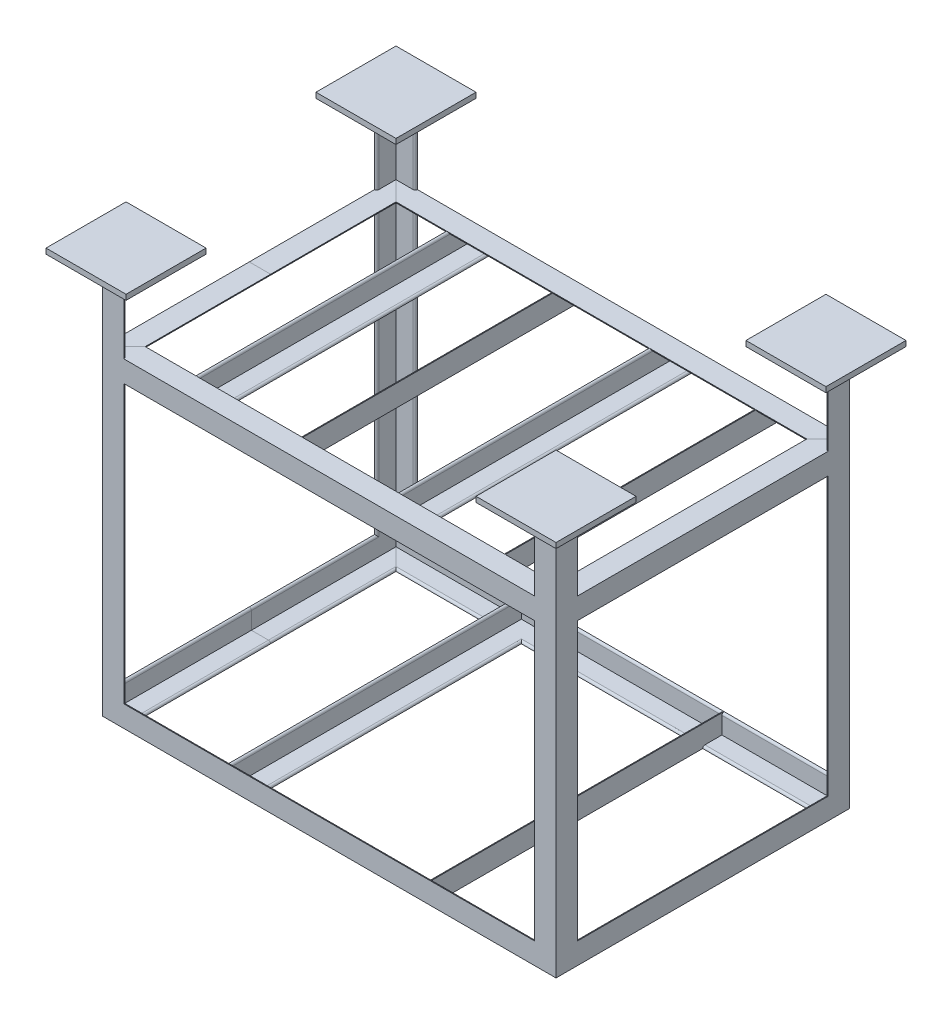
from build123d import *

# Parameters (mm, degrees)
BOSS_EXTRUDE_1_DEPTH = 300
BOSS_EXTRUDE_START   = 150
BOSS_EXTRUDE_2_DEPTH = 150
SKETCH_4_W           = 150
SKETCH_4_H           = 150
BOSS_EXTRUDE_3_DEPTH = 10
BOSS_EXTRUDE_4_REACH = 977.753


with BuildPart() as part:
    # Sweep 1: sweep along a path in Sketch 1
    with BuildLine(Plane(origin=(0, 0, 0), x_dir=(1, 0, 0), z_dir=(0, 1, 0))) as sweep_1_path:
        Line((-425, -275), (-425, 275))
        Line((-425, 275), (425, 275))
        Line((425, 275), (425, -275))
        Line((425, -275), (-425, -275))
    # Sketch 2 → Sweep 1 (sweep)
    with BuildSketch(Plane.XY):
        with BuildLine():
            Line((-425, 0), (-385, 0))
            ThreePointArc((-385, 0), (-386.171572875, -2.828427125), (-389, -4))
            Line((-389, -4), (-421, -4))
            Line((-421, -4), (-421, -36))
            ThreePointArc((-421, -36), (-422.171572875, -38.828427125), (-425, -40))
            Line((-425, -40), (-425, 0))
        make_face()
    sweep(path=sweep_1_path.line, transition=Transition.RIGHT)

    # Sketch 3_2 → Boss-Extrude 1 (add)
    with BuildSketch(Plane(origin=(0, 0, 0), x_dir=(1, 0, 0), z_dir=(0, 1, 0))):
        with BuildLine():
            Line((425, 275), (425, 235))
            ThreePointArc((425, 235), (422.171572875, 236.171572875), (421, 239))
            Line((421, 239), (421, 271))
            Line((421, 271), (389, 271))
            ThreePointArc((389, 271), (386.171572875, 272.171572875), (385, 275))
            Line((385, 275), (425, 275))
        make_face()
        with BuildLine():
            Line((425, -275), (385, -275))
            ThreePointArc((385, -275), (386.171572875, -272.171572875), (389, -271))
            Line((389, -271), (421, -271))
            Line((421, -271), (421, -239))
            ThreePointArc((421, -239), (422.171572875, -236.171572875), (425, -235))
            Line((425, -235), (425, -275))
        make_face()
        with BuildLine():
            Line((-425, -275), (-425, -235))
            ThreePointArc((-425, -235), (-422.171572875, -236.171572875), (-421, -239))
            Line((-421, -239), (-421, -271))
            Line((-421, -271), (-389, -271))
            ThreePointArc((-389, -271), (-386.171572875, -272.171572875), (-385, -275))
            Line((-385, -275), (-425, -275))
        make_face()
        with BuildLine():
            Line((-425, 275), (-385, 275))
            ThreePointArc((-385, 275), (-386.171572875, 272.171572875), (-389, 271))
            Line((-389, 271), (-421, 271))
            Line((-421, 271), (-421, 239))
            ThreePointArc((-421, 239), (-422.171572875, 236.171572875), (-425, 235))
            Line((-425, 235), (-425, 275))
        make_face()
    extrude(amount=-BOSS_EXTRUDE_1_DEPTH)

    # Mirror 4: part across plane


with BuildPart() as part_1:
    add(part.part)
    add(part.part.mirror(Plane(origin=(389, -300, -275), x_dir=(0, 0, 1), z_dir=(0, -1, 0))))

    # Sketch 3_2 2 → Boss-Extrude 2 (add)
    with BuildSketch(Plane(origin=(0, 0, 0), x_dir=(1, 0, 0), z_dir=(0, 1, 0)).offset(BOSS_EXTRUDE_START)):
        with BuildLine():
            Line((425, 275), (425, 235))
            ThreePointArc((425, 235), (422.171572875, 236.171572875), (421, 239))
            Line((421, 239), (421, 271))
            Line((421, 271), (389, 271))
            ThreePointArc((389, 271), (386.171572875, 272.171572875), (385, 275))
            Line((385, 275), (425, 275))
        make_face()
        with BuildLine():
            Line((425, -275), (385, -275))
            ThreePointArc((385, -275), (386.171572875, -272.171572875), (389, -271))
            Line((389, -271), (421, -271))
            Line((421, -271), (421, -239))
            ThreePointArc((421, -239), (422.171572875, -236.171572875), (425, -235))
            Line((425, -235), (425, -275))
        make_face()
        with BuildLine():
            Line((-425, -275), (-425, -235))
            ThreePointArc((-425, -235), (-422.171572875, -236.171572875), (-421, -239))
            Line((-421, -239), (-421, -271))
            Line((-421, -271), (-389, -271))
            ThreePointArc((-389, -271), (-386.171572875, -272.171572875), (-385, -275))
            Line((-385, -275), (-425, -275))
        make_face()
        with BuildLine():
            Line((-425, 275), (-385, 275))
            ThreePointArc((-385, 275), (-386.171572875, 272.171572875), (-389, 271))
            Line((-389, 271), (-421, 271))
            Line((-421, 271), (-421, 239))
            ThreePointArc((-421, 239), (-422.171572875, 236.171572875), (-425, 235))
            Line((-425, 235), (-425, 275))
        make_face()
    extrude(amount=-BOSS_EXTRUDE_2_DEPTH)

    # Sketch 4 → Boss-Extrude 3 (add)
    with BuildSketch(Plane(origin=(0, 150, 0), x_dir=(1, 0, 0), z_dir=(0, 1, 0))):
        with Locations((403, -253)):
            Rectangle(SKETCH_4_W, SKETCH_4_H)
        with Locations((403, 253)):
            Rectangle(SKETCH_4_W, SKETCH_4_H)
        with Locations((-403, 253)):
            Rectangle(SKETCH_4_W, SKETCH_4_H)
        with Locations((-403, -253)):
            Rectangle(SKETCH_4_W, SKETCH_4_H)
    extrude(amount=BOSS_EXTRUDE_3_DEPTH)

    # Sketch 5 → Boss-Extrude 4 (add, up to next)
    with BuildSketch(Plane.XY.offset(275), mode=Mode.PRIVATE) as boss_extrude_4_sk1:
        with BuildLine():
            Line((290, 0), (290, -40))
            Line((290, -40), (250, -40))
            ThreePointArc((250, -40), (251.171572875, -37.171572875), (254, -36))
            Line((254, -36), (286, -36))
            Line((286, -36), (286, -4))
            ThreePointArc((286, -4), (287.171572875, -1.171572875), (290, 0))
        make_face()
    boss_extrude_4_tool1 = extrude(boss_extrude_4_sk1.sketch, amount=-BOSS_EXTRUDE_4_REACH, mode=Mode.PRIVATE) - part_1.part
    # Sketch 5 → Boss-Extrude 4 (add, up to next)
    with BuildSketch(Plane.XY.offset(275), mode=Mode.PRIVATE) as boss_extrude_4_sk2:
        with BuildLine():
            Line((130, -40), (90, -40))
            Line((90, -40), (90, 0))
            ThreePointArc((90, 0), (92.828427125, -1.171572875), (94, -4))
            Line((94, -4), (94, -36))
            Line((94, -36), (126, -36))
            ThreePointArc((126, -36), (128.828427125, -37.171572875), (130, -40))
        make_face()
    boss_extrude_4_tool2 = extrude(boss_extrude_4_sk2.sketch, amount=-BOSS_EXTRUDE_4_REACH, mode=Mode.PRIVATE) - part_1.part
    # Sketch 5 → Boss-Extrude 4 (add, up to next)
    with BuildSketch(Plane.XY.offset(275), mode=Mode.PRIVATE) as boss_extrude_4_sk3:
        with BuildLine():
            Line((-90, 0), (-90, -40))
            Line((-90, -40), (-130, -40))
            ThreePointArc((-130, -40), (-128.828427125, -37.171572875), (-126, -36))
            Line((-126, -36), (-94, -36))
            Line((-94, -36), (-94, -4))
            ThreePointArc((-94, -4), (-92.828427125, -1.171572875), (-90, 0))
        make_face()
    boss_extrude_4_tool3 = extrude(boss_extrude_4_sk3.sketch, amount=-BOSS_EXTRUDE_4_REACH, mode=Mode.PRIVATE) - part_1.part
    # Sketch 5 → Boss-Extrude 4 (add, up to next)
    with BuildSketch(Plane.XY.offset(275), mode=Mode.PRIVATE) as boss_extrude_4_sk4:
        with BuildLine():
            Line((-250, -40), (-290, -40))
            Line((-290, -40), (-290, 0))
            ThreePointArc((-290, 0), (-287.171572875, -1.171572875), (-286, -4))
            Line((-286, -4), (-286, -36))
            Line((-286, -36), (-254, -36))
            ThreePointArc((-254, -36), (-251.171572875, -37.171572875), (-250, -40))
        make_face()
    boss_extrude_4_tool4 = extrude(boss_extrude_4_sk4.sketch, amount=-BOSS_EXTRUDE_4_REACH, mode=Mode.PRIVATE) - part_1.part
    # Sketch 5 → Boss-Extrude 4 (add, up to next)
    with BuildSketch(Plane.XY.offset(275), mode=Mode.PRIVATE) as boss_extrude_4_sk5:
        with BuildLine():
            Line((150, -600), (190, -600))
            Line((190, -600), (190, -560))
            ThreePointArc((190, -560), (187.171572875, -561.171572875), (186, -564))
            Line((186, -564), (186, -596))
            Line((186, -596), (154, -596))
            ThreePointArc((154, -596), (151.171572875, -597.171572875), (150, -600))
        make_face()
    boss_extrude_4_tool5 = extrude(boss_extrude_4_sk5.sketch, amount=-BOSS_EXTRUDE_4_REACH, mode=Mode.PRIVATE) - part_1.part
    # Sketch 5 → Boss-Extrude 4 (add, up to next)
    with BuildSketch(Plane.XY.offset(275), mode=Mode.PRIVATE) as boss_extrude_4_sk6:
        with BuildLine():
            Line((-190, -560), (-190, -600))
            Line((-190, -600), (-150, -600))
            ThreePointArc((-150, -600), (-151.171572875, -597.171572875), (-154, -596))
            Line((-154, -596), (-186, -596))
            Line((-186, -596), (-186, -564))
            ThreePointArc((-186, -564), (-187.171572875, -561.171572875), (-190, -560))
        make_face()
    boss_extrude_4_tool6 = extrude(boss_extrude_4_sk6.sketch, amount=-BOSS_EXTRUDE_4_REACH, mode=Mode.PRIVATE) - part_1.part
    add(boss_extrude_4_tool1.solids().sort_by_distance((289.434315, -20, 275))[0])
    add(boss_extrude_4_tool2.solids().sort_by_distance((110, -39.434315, 275))[0])
    add(boss_extrude_4_tool3.solids().sort_by_distance((-90.565685, -20, 275))[0])
    add(boss_extrude_4_tool4.solids().sort_by_distance((-251.571573, -37.571573, 275))[0])
    add(boss_extrude_4_tool5.solids().sort_by_distance((170, -599.434315, 275))[0])
    add(boss_extrude_4_tool6.solids().sort_by_distance((-187.571573, -561.571573, 275))[0])


solid = part_1.part
